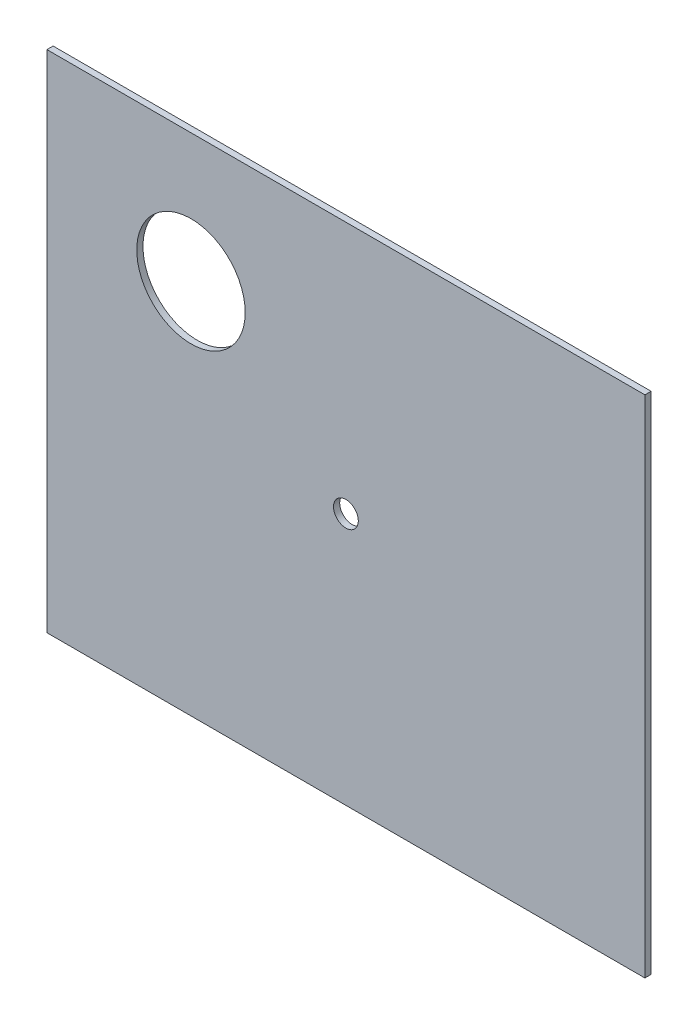
from build123d import *

# Parameters (mm, degrees)
SKETCH_1_W          = 386
SKETCH_1_H          = 326
EXTRUDE_1_DEPTH     = 2
SKETCH_2_R          = 8
SKETCH_2_R_2        = 35
CUT_EXTRUDE_1_DEPTH = 12


with BuildPart() as part:
    # 草图1 → 凸台-拉伸1 (new, symmetric)
    with BuildSketch(Plane.XY):
        Rectangle(SKETCH_1_W, SKETCH_1_H)
    extrude(amount=EXTRUDE_1_DEPTH, both=True)

    # 草图2 → 切除-拉伸1 (cut, symmetric)
    with BuildSketch(Plane.XY):
        Circle(SKETCH_2_R)
        with Locations((-100, 80)):
            Circle(SKETCH_2_R_2)
    extrude(amount=CUT_EXTRUDE_1_DEPTH, both=True, mode=Mode.SUBTRACT)


solid = part.part
